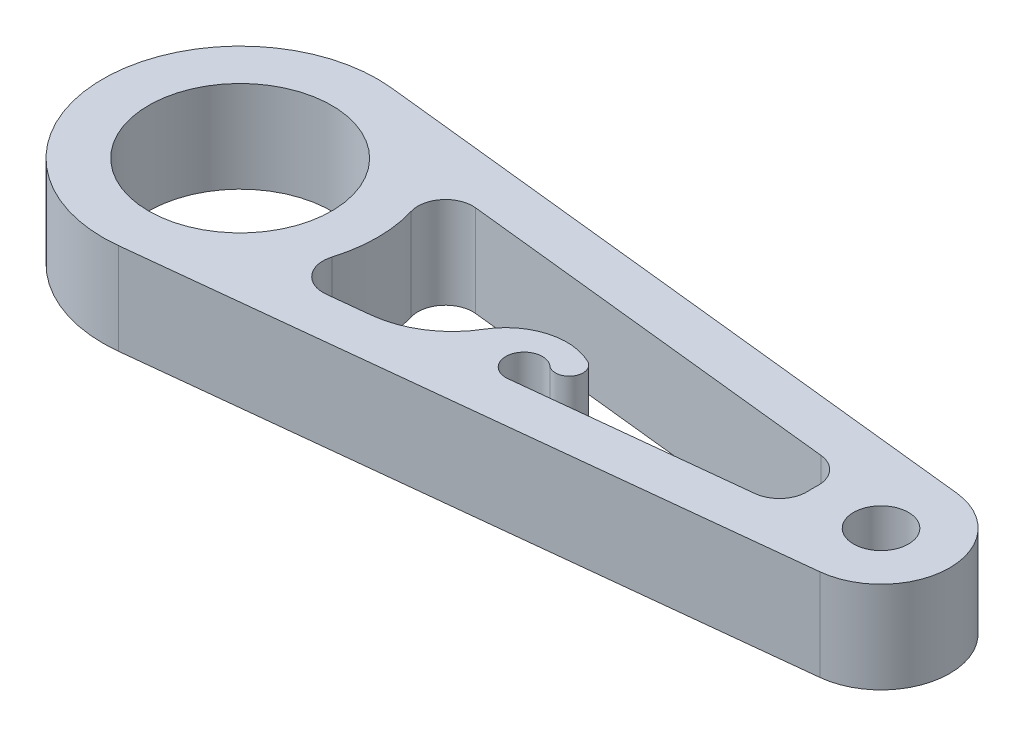
from build123d import *

# Parameters (mm, degrees)
SKETCH_1_R      = 10
SKETCH_1_R_2    = 3
EXTRUDE_1_DEPTH = 10
FILLET_1_R      = 3
EXTRUDE_3_DEPTH = 10
FILLET_3_R      = 10


with BuildPart() as part:
    # 草图1 → 凸台-拉伸1 (new body)
    with BuildSketch(Plane(origin=(0, 0, 0), x_dir=(1, 0, 0), z_dir=(0, 1, 0))):
        with BuildLine():
            Line((1.607142857, 14.913654543), (70.803571429, 7.456827272))
            ThreePointArc((70.803571429, 7.456827272), (77.5, 0), (70.803571429, -7.456827272))
            Line((70.803571429, -7.456827272), (1.607142857, -14.913654543))
            ThreePointArc((1.607142857, -14.913654543), (-15, 0), (1.607142857, 14.913654543))
        make_face()
        with Locations(Location((0, 0, 0), (0, 0, 270))):
            Circle(SKETCH_1_R, mode=Mode.SUBTRACT)
        with Locations(Location((70, 0, 0), (0, 0, 270))):
            Circle(SKETCH_1_R_2, mode=Mode.SUBTRACT)
        with BuildLine():
            Line((12.187410355, 8.744542803), (63.23749297, 3.243223499))
            ThreePointArc((63.23749297, 3.243223499), (62.5, 0), (63.23749297, -3.243223499))
            Line((63.23749297, -3.243223499), (12.187410355, -8.744542803))
            ThreePointArc((12.187410355, -8.744542803), (15, 0), (12.187410355, 8.744542803))
        make_face(mode=Mode.SUBTRACT)
    extrude(amount=EXTRUDE_1_DEPTH)

    # 圆角1
    fillet_1_edges = [part.edges().sort_by_distance(p)[0] for p in [
        (12.187410355, 5, -8.744542803),
        (12.187410355, 5, 8.744542803),
        (63.23749297, 5, 3.243223499),
        (63.23749297, 5, -3.243223499),
    ]]
    fillet(fillet_1_edges, radius=FILLET_1_R)

    # 草图3 → 凸台-拉伸3 (add)
    with BuildSketch(Plane(origin=(0, 10, 0), x_dir=(1, 0, 0), z_dir=(0, 1, 0))):
        with BuildLine():
            Line((28.613097425, -6.974458511), (35.472880926, -6.235226418))
            ThreePointArc((35.472880926, -6.235226418), (33.348074169, -3.655207792), (36.559018282, -2.727232699))
            ThreePointArc((36.559018282, -2.727232699), (38.788114159, -2.411034272), (38.192669869, -0.239791316))
            ThreePointArc((38.192669869, -0.239791316), (31.413780396, -0.777770747), (28.613097425, -6.974458511))
        make_face()
    extrude(amount=-EXTRUDE_3_DEPTH)

    # 圆角3
    fillet_3_edges = [part.edges().sort_by_distance(p)[0] for p in [
        (28.613097425, 5, 6.974458511),
    ]]
    fillet(fillet_3_edges, radius=FILLET_3_R)


solid = part.part
